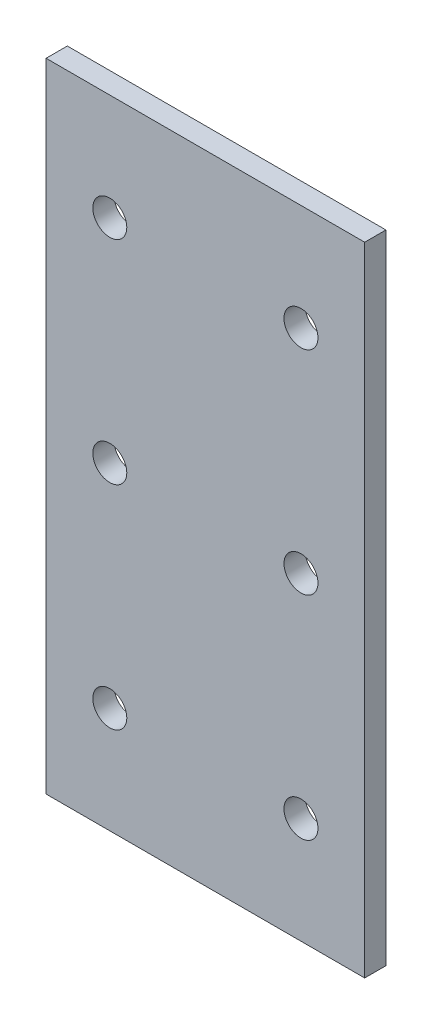
from build123d import *

# Parameters (mm, degrees)
SKETCH1_W           = 150
SKETCH1_H           = 300
SKETCH1_R           = 8
BOSS_EXTRUDE1_DEPTH = 10


with BuildPart() as part:
    # Sketch1 → Boss-Extrude1 (new body)
    with BuildSketch(Plane.XY):
        Rectangle(SKETCH1_W, SKETCH1_H)
        with Locations((-45, 100)):
            Circle(SKETCH1_R, mode=Mode.SUBTRACT)
        with Locations((-45, 0)):
            Circle(SKETCH1_R, mode=Mode.SUBTRACT)
        with Locations((-45, -100)):
            Circle(SKETCH1_R, mode=Mode.SUBTRACT)
        with Locations(Location((45, -100, 0), (0, 0, 180))):
            Circle(SKETCH1_R, mode=Mode.SUBTRACT)
        with Locations(Location((45, 0, 0), (0, 0, 180))):
            Circle(SKETCH1_R, mode=Mode.SUBTRACT)
        with Locations(Location((45, 100, 0), (0, 0, 180))):
            Circle(SKETCH1_R, mode=Mode.SUBTRACT)
    extrude(amount=BOSS_EXTRUDE1_DEPTH)


solid = part.part
